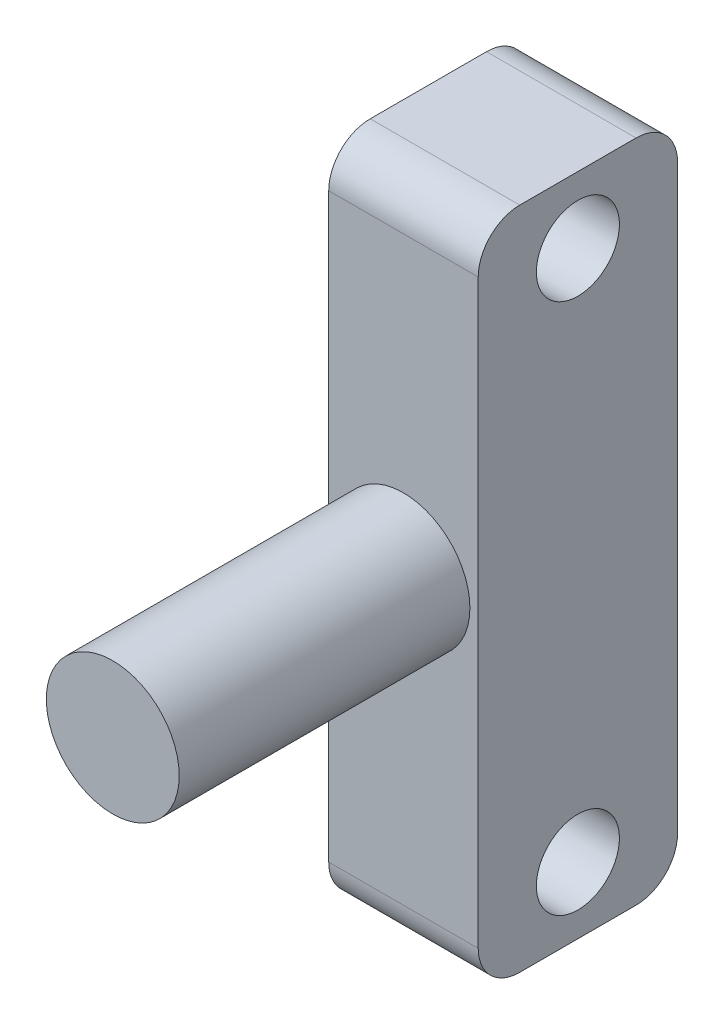
SolidWorks part; units mm, degrees
ref_plane "Front Plane" through (0, 0, 0) normal (0, 0, 1) x (1, 0, 0)
ref_plane "Top Plane" through (0, 0, 0) normal (0, 1, 0) x (1, 0, 0)
ref_plane "Right Plane" through (0, 0, 0) normal (1, 0, 0) x (0, 0, -1)
sketch "Sketch1" plane through (0, 0, 0) normal (0, 0, 1) x (1, 0, 0)
  circle A0 centre (0, 0) radius 8
  dimension "D1" = 16
extrude "Boss-Extrude1" add sketch "Sketch1" along normal blind 35
sketch "Sketch2" plane through (0, 0, 0) normal (0, 0, -1) x (-1, 0, 0)
  line L1 (9, 40) -> (-9, 40)
  line L2 (9, 40) -> (9, -40)
  line L3 (9, -40) -> (-9, -40)
  line L4 (-9, 40) -> (-9, -40)
  line L5 (9, 40) -> (-9, -40) construction
  line L6 (9, -40) -> (-9, 40) construction
  point P0 (0, 0)
  dimension "D1" = 18
  dimension "D2" = 80
extrude "Boss-Extrude2" add sketch "Sketch2" along normal blind 24
fillet "Fillet1" radius 5 4 edges at (0, -40, 0) (0, -40, -24) (0, 40, 0) (0, 40, -24)
sketch "Sketch4" plane through (-9, 0, 0) normal (-1, 0, 0) x (0, 0, 1)
  line L0 (-12, 40) -> (-12, -40) construction
  line L1 (-19, 40) -> (-5, 40) construction
  line L2 (-19, -40) -> (-5, -40) construction
  circle A0 centre (-12, -32) radius 5
  circle A1 centre (-12, 32) radius 5
  dimension "D3" = 10
  dimension "D4" = 10
  dimension "D1" = 64
  dimension "D2" = 32
extrude "Cut-Extrude1" cut sketch "Sketch4" against normal through all
